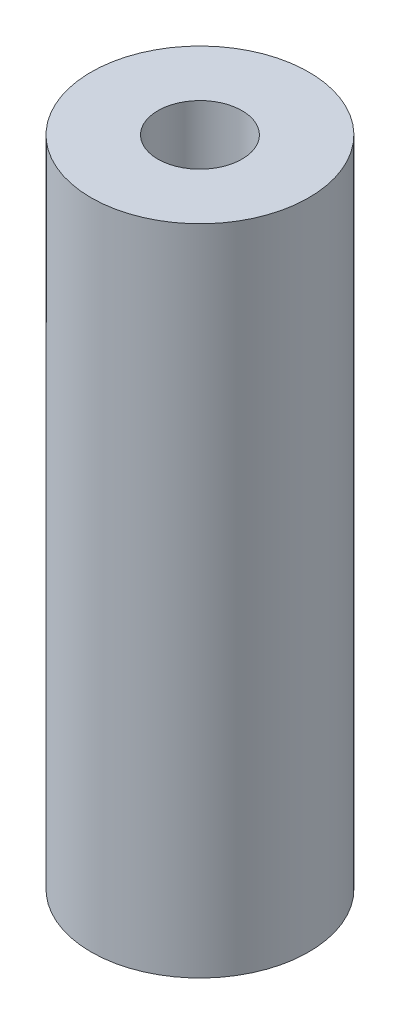
SolidWorks part; units mm, degrees
material "SS400B"
ref_plane "Front Plane" through (0, 0, 0) normal (0, 0, 1) x (1, 0, 0)
ref_plane "Top Plane" through (0, 0, 0) normal (0, 1, 0) x (1, 0, 0)
ref_plane "Right Plane" through (0, 0, 0) normal (1, 0, 0) x (0, 0, -1)
sketch "Sketch1" plane through (0, 0, 0) normal (0, 1, 0) x (1, 0, 0)
  circle A0 centre (0, 0) radius 11
  dimension "D1" = 22
extrude "Boss-Extrude1" add sketch "Sketch1" along normal blind 66
hole_wizard "M10 Tapped Hole1" positions "Sketch3" profile "Sketch4" tap size "M10" standard "GB"
sketch "Sketch3" plane through (0, 66, 0) normal (0, 1, 0) x (1, 0, 0)
  point P0 (0, 0)
sketch "Sketch4" plane through (0, 66, 0) normal (1, 0, 0) x (0, 0, 1)
  line L0 (0, 0) -> (0, 27.5537)
  line L1 (0, 27.5537) -> (4.25, 25)
  line L2 (4.25, 25) -> (4.25, 0)
  line L5 (4.25, 0) -> (0, 0)
  line L10 (0, 27.5537) -> (-4.25, 25) construction
  line L11 (0, -6.35) -> (0, 107.95) construction
  dimension "螺纹孔钻头直径" = 8.5
  dimension "螺纹孔钻头深度" = 25
  dimension "导头角度" = 118
cosmetic thread "Cosmetic Thread1" parameters "D1"=20, "D2"=10
